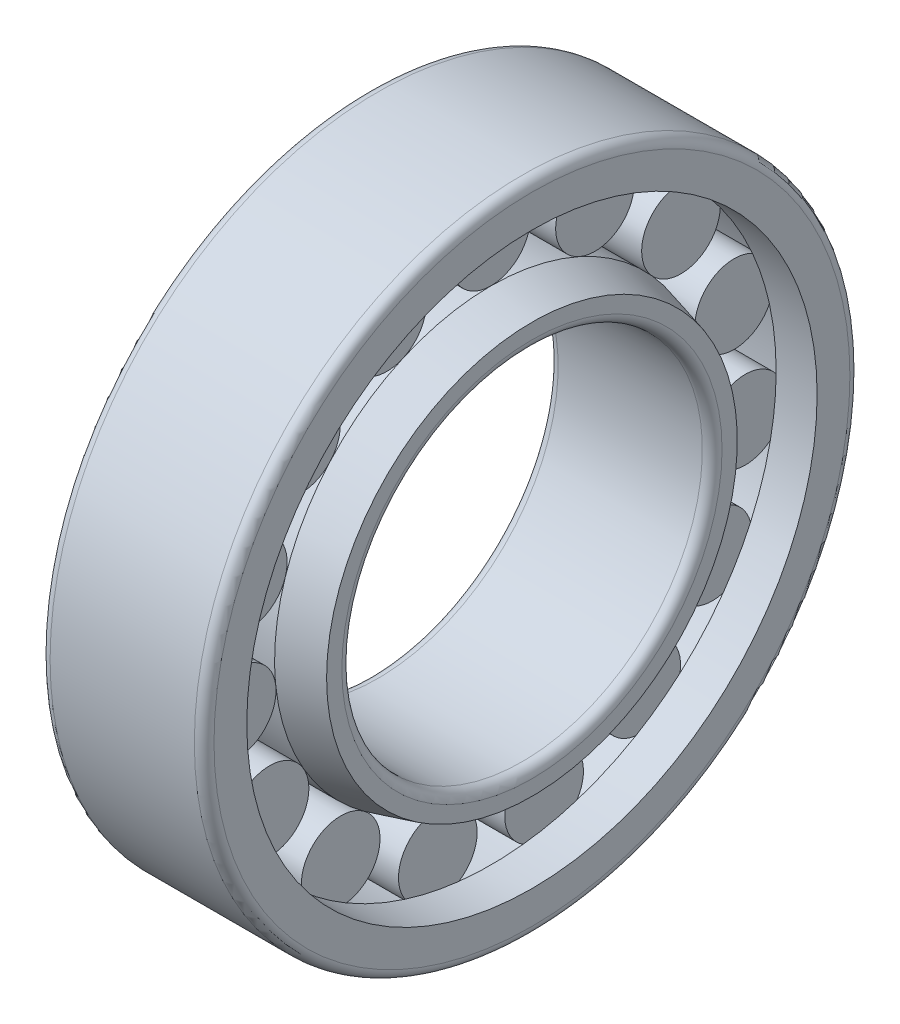
SolidWorks part; units mm, degrees
revolve "Base-Revolve" add sketch "Sketch2" angle 360 about L0
sketch "Sketch2" plane through (0, 0, 0) normal (0, 0, 1) x (1, 0, 0)
  line L0 (-10.0801, 0) -> (21.9267, 0) construction
  line L1 (6.25, 33) -> (18.75, 33)
  line L2 (0, 29.4783) -> (6.25, 33)
  line L3 (0, 29.4783) -> (0, 29)
  line L4 (1.5, 27.5) -> (23.5, 27.5)
  line L5 (25, 31.3253) -> (25, 29)
  line L7 (25, 31.3253) -> (18.75, 33)
  arc A0 (23.5, 27.5) -> (25, 29) centre (23.5, 29) ccw
  arc A1 (0, 29) -> (1.5, 27.5) centre (1.5, 29) ccw
  point P13 (25, 27.5)
  point P16 (0, 27.5)
material "GCr15SiMn"
ref_plane "Plane1" through (0, 0, 0) normal (0, 0, 1) x (1, 0, 0)
ref_plane "Plane2" through (0, 0, 0) normal (0, 1, 0) x (1, 0, 0)
ref_plane "Plane3" through (0, 0, 0) normal (1, 0, 0) x (0, 0, -1)
sketch "Sketch dimensions" plane through (0, 0, 0) normal (0, 0, 1) x (1, 0, 0)
  line L0 (0, 0) -> (1.5, 0)
  line L1 (1.5, 0) -> (3, 0)
  line L2 (3, 0) -> (28, 0)
  line L3 (28, 0) -> (83, 0)
  line L4 (83, 0) -> (149, 0)
  line L5 (149, 0) -> (249, 0)
  line L7 (249, 0) -> (339, 0)
sketch "Sketch3" plane through (0, 0, 0) normal (0, 0, 1) x (1, 0, 0)
  line L0 (6.25, 33) -> (6.25, -33) construction
  line L1 (18.75, 33) -> (18.75, -33) construction
  line L2 (-1.6039, 39) -> (13.5036, 39) construction
  line L4 (6.25, 39) -> (18.75, 39)
  line L5 (6.25, 39) -> (6.25, 32.9999)
  line L6 (6.25, 32.9999) -> (18.75, 32.9999)
  line L7 (18.75, 39) -> (18.75, 32.9999)
revolve "Boss-Revolve1" add sketch "Sketch3" angle 360 about L2
sketch "Sketch4" plane through (0, 0, 0) normal (0, 0, 1) x (1, 0, 0)
  line L0 (0, 0) -> (17.8006, 0) construction
  line L1 (-10.0801, 0) -> (21.9267, 0) construction
  line L2 (18.75, 43.5) -> (25, 43.5)
  line L3 (1.5, 50) -> (23.5, 50)
  line L4 (0, 48.5) -> (0, 43.5)
  line L5 (0, 43.5) -> (6.25, 43.5)
  line L6 (25, 48.5) -> (25, 43.5)
  line L7 (6.25, 45) -> (18.75, 45)
  line L8 (6.25, 45) -> (6.25, 43.5)
  line L10 (18.75, 45) -> (18.75, 43.5)
  arc A0 (23.5, 50) -> (25, 48.5) centre (23.5, 48.5) cw
  arc A1 (1.5, 50) -> (0, 48.5) centre (1.5, 48.5) ccw
  point P15 (25, 50)
  point P18 (0, 50)
revolve "Boss-Revolve2" add sketch "Sketch4" angle 360 about L0
pattern_circular "CirPattern1" count 15 over 360 about axis through (0, 0, 0) along (1, 0, 0) of "Boss-Revolve1"
equation "\"DD@Sketch2\" = \"内径@Sketch dimensions\""
equation "\"FW@Sketch2\" = \"参考FW@Sketch dimensions\""
equation "\"D1@Sketch2\" = \"倒角小@Sketch dimensions\""
equation "\"EW@Sketch4\" = \"参考EW@Sketch dimensions\""
equation "\"D@Sketch4\" = \"外径@Sketch dimensions\""
equation "\"D2@Sketch4\" = \"倒角大@Sketch dimensions\""
equation "\"B@Sketch4\" = \"宽度@Sketch dimensions\""
equation "\"D1@Sketch3\" =  ( \"EW@Sketch4\" - \"FW@Sketch2\" )  / 4 + \"FW@Sketch2\" / 2"
equation "\"D2@Sketch3\" =  0.25*( \"EW@Sketch4\" - \"FW@Sketch2\" ) +0.0001"
equation "\"D2@Sketch2\" = \"B@Sketch4\""
equation "\"D4@Sketch2\" = \"FW@Sketch2\" + 4 *\"D1@Sketch2\""
equation "\"滚珠位置@Sketch2\" = \"D2@Sketch2\"/4"
equation "\"D3@Sketch4\" = \"D2@Sketch4\""
equation "\"D1@CirPattern1\" = 0.75*\"D1@Sketch3\" * 3.14 / \"D2@Sketch3\""
